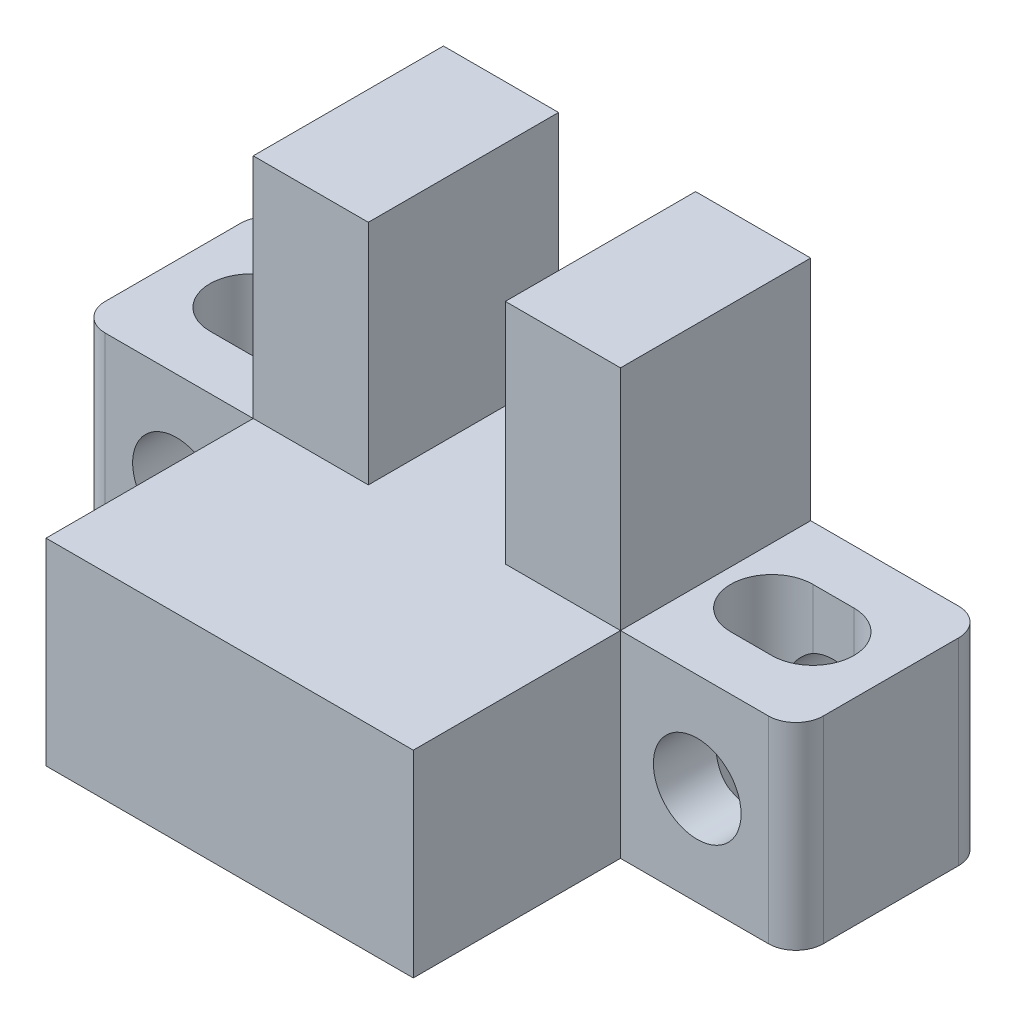
SolidWorks part; units mm, degrees
ref_plane "Front" through (0, 0, 0) normal (0, 0, 1) x (1, 0, 0)
ref_plane "Top" through (0, 0, 0) normal (0, 1, 0) x (1, 0, 0)
ref_plane "Right" through (0, 0, 0) normal (1, 0, 0) x (0, 0, -1)
sketch "草图1" plane through (0, 0, 0) normal (0, 1, 0) x (1, 0, 0)
  line L0 (0, -6.94) -> (6.4, -6.94)
  line L1 (0, 0) -> (26.2, 0)
  line L2 (0, 0) -> (0, -6.94)
  line L3 (6.4, -14.5) -> (19.8, -14.5)
  line L4 (26.2, 0) -> (26.2, -6.94)
  line L5 (6.4, -6.94) -> (6.4, -14.5)
  line L6 (26.2, -6.94) -> (19.8, -6.94)
  line L7 (19.8, -6.94) -> (19.8, -14.5)
  dimension "D1" = 26.2
  dimension "D2" = 14.5
  dimension "D3" = 13.4
  dimension "D4" = 6.94
extrude "凸台-拉伸1" add sketch "草图1" along normal blind 7.2
sketch "草图2" plane through (0, 7.2, 0) normal (0, 1, 0) x (1, 0, 0)
  line L0 (26.2, 0) -> (0, 0) construction
  line L1 (6.4, -6.94) -> (10.6, -6.94)
  line L2 (6.4, -6.94) -> (6.4, 0)
  line L3 (6.4, 0) -> (10.6, 0)
  line L4 (19.8, -6.94) -> (19.8, 0)
  line L5 (10.6, 0) -> (10.6, -6.94)
  line L6 (15.6, 0) -> (15.6, -6.94)
  line L7 (15.6, -6.94) -> (19.8, -6.94)
  line L8 (15.6, 0) -> (19.8, 0)
  dimension "D1" = 13.4
  dimension "D2" = 5
extrude "凸台-拉伸2" add sketch "草图2" along normal blind 8.3
sketch "草图3" plane through (0, 7.2, 0) normal (0, 1, 0) x (1, 0, 0)
  line L0 (2.85, -3.47) -> (4.35, -3.47) construction
  line L1 (2.85, -1.97) -> (4.35, -1.97)
  line L2 (2.85, -4.97) -> (4.35, -4.97)
  line L3 (23.35, -3.47) -> (21.85, -3.47) construction
  line L4 (23.35, -4.97) -> (21.85, -4.97)
  line L5 (23.35, -1.97) -> (21.85, -1.97)
  line L6 (26.2, 0) -> (19.8, 0) construction
  line L8 (26.2, 0) -> (0, 0) construction
  arc A0 (2.85, -1.97) -> (2.85, -4.97) centre (2.85, -3.47) ccw
  arc A1 (4.35, -4.97) -> (4.35, -1.97) centre (4.35, -3.47) ccw
  arc A2 (23.35, -4.97) -> (23.35, -1.97) centre (23.35, -3.47) ccw
  arc A3 (21.85, -1.97) -> (21.85, -4.97) centre (21.85, -3.47) ccw
  point P2 (3.6, -3.47)
  point P9 (22.6, -3.47)
  point P16 (13.1, 0)
  dimension "D1" = 3.47
  dimension "D2" = 1.5
  dimension "D3" = 19
  dimension "D4" = 9.5
  dimension "D5" = 3
extrude "切除-拉伸1" cut sketch "草图3" against normal through all
sketch "草图4" plane through (0, 0, 6.94) normal (0, 0, 1) x (1, 0, 0)
  line L0 (19.8, 0) -> (26.2, 0) construction
  line L2 (6.4, 7.2) -> (19.8, 7.2) construction
  circle A0 centre (22.6, 3.6) radius 1.6
  circle A1 centre (3.6, 3.6) radius 1.6
  point P8 (13.1, 7.2)
  dimension "D1" = 3.2
  dimension "D2" = 3.6
  dimension "D3" = 19
  dimension "D4" = 9.5
extrude "切除-拉伸2" cut sketch "草图4" against normal through all
fillet "圆角1" radius 1 4 edges at (0, 3.6, 0) (0, 3.6, 6.94) (26.2, 3.6, 0) (26.2, 3.6, 6.94)
